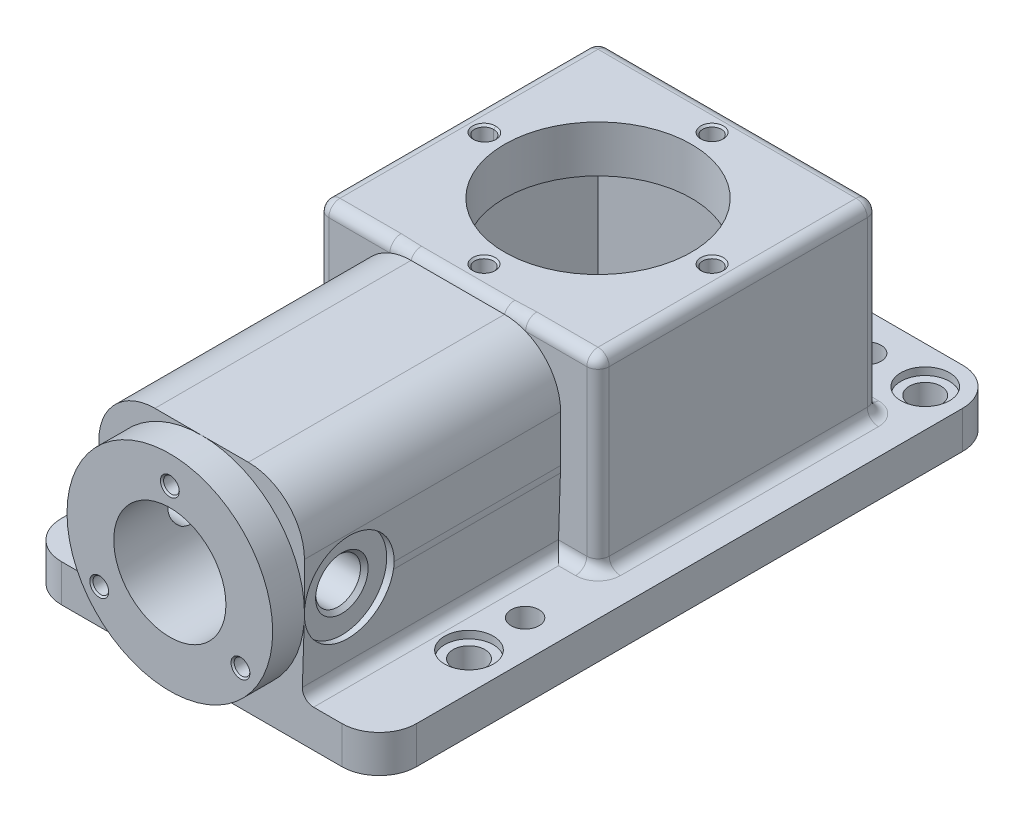
from build123d import *

# Parameters (mm, degrees)
SKETCH1_R                       = 27.5
BOSS_EXTRUDE1_DEPTH             = 77
SKETCH2_W                       = 75
SKETCH2_H                       = 56.897365196
BOSS_EXTRUDE2_DEPTH             = 75
SKETCH3_R                       = 15
CUT_EXTRUDE1_DEPTH              = 105
SKETCH4_R                       = 25
CUT_EXTRUDE2_DEPTH              = 17
SKETCH5_R                       = 21
CUT_EXTRUDE3_DEPTH              = 65
CUT_EXTRUDE4_START              = -12.5
SKETCH6_W                       = 63
SKETCH6_H                       = 63
CUT_EXTRUDE4_DEPTH              = 39.5
SKETCH7_R                       = 25
SKETCH7_R_2                     = 21
BOSS_EXTRUDE3_DEPTH             = 2
BOSS_EXTRUDE4_DEPTH             = 47.5
BOSS_EXTRUDE5_START             = -68.5
BOSS_EXTRUDE5_DEPTH             = 68.5
FILLET1_R                       = 15
FILLET2_R                       = 3
BOSS_EXTRUDE7_REACH             = 124.474
SKETCH19_W                      = 17.5
SKETCH19_H                      = 130
SKETCH20_W                      = 148
SKETCH20_H                      = 3.566
CUT_EXTRUDE9_DEPTH              = 205
SKETCH10_R                      = 6.5
CUT_EXTRUDE5_DEPTH              = 2
SKETCH11_R                      = 4.25
CUT_EXTRUDE6_DEPTH              = 69
FILLET3_R                       = 10
SKETCH12_R                      = 21
CUT_EXTRUDE7_DEPTH              = 69
BOSS_EXTRUDE6_START             = 2
SKETCH13_R                      = 25
SKETCH13_R_2                    = 21
BOSS_EXTRUDE6_DEPTH             = 2
CIRPATTERN1_COUNT               = 3
SKETCH16_R                      = 3.735111871
SKETCH16_R_2                    = 3.711892177
CUT_EXTRUDE8_DEPTH              = 25
FILLET4_R                       = 3
SKETCH22_R                      = 12
CUT_EXTRUDE10_DEPTH             = 2
M6_TAPPED_HOLE1_D               = 5
M6_TAPPED_HOLE1_DEPTH           = 9.497848452
M6_TAPPED_HOLE1_CSINK_D         = 6.05
M6_TAPPED_HOLE1_CSINK_ANGLE     = 90
M6_TAPPED_HOLE1_TIP             = 1.502151548
SKETCH30_R                      = 7
CUT_EXTRUDE11_DEPTH             = 1
M8X1_0_TAPPED_HOLE1_D           = 7
M8X1_0_TAPPED_HOLE1_DEPTH       = 16.896987833
M8X1_0_TAPPED_HOLE1_CSINK_D     = 8.05
M8X1_0_TAPPED_HOLE1_CSINK_ANGLE = 90
M8X1_0_TAPPED_HOLE1_TIP         = 2.103012167


with BuildPart() as part:
    # Sketch1 → Boss-Extrude1 (new body)
    with BuildSketch(Plane.XY):
        Circle(SKETCH1_R)
    extrude(amount=BOSS_EXTRUDE1_DEPTH)

    # Sketch2 → Boss-Extrude2 (add)
    with BuildSketch(Plane(origin=(0, 0, 0), x_dir=(-1, 0, 0), z_dir=(0, 0, -1))):
        with Locations((0, 0.948682598)):
            Rectangle(SKETCH2_W, SKETCH2_H)
    extrude(amount=BOSS_EXTRUDE2_DEPTH)

    # Sketch3 → Cut-Extrude1 (cut)
    with BuildSketch(Plane.XY.offset(77)):
        Circle(SKETCH3_R)
    extrude(amount=-CUT_EXTRUDE1_DEPTH, mode=Mode.SUBTRACT)

    # Sketch4 → Cut-Extrude2 (cut)
    with BuildSketch(Plane(origin=(0, 29.397365196, 0), x_dir=(1, 0, 0), z_dir=(0, 1, 0))):
        with Locations(Location((0, 37.5, 0), (0, 0, 180))):
            Circle(SKETCH4_R)
    extrude(amount=-CUT_EXTRUDE2_DEPTH, mode=Mode.SUBTRACT)

    # Sketch5 → Cut-Extrude3 (cut)
    with BuildSketch(Plane.XZ.offset(27.5)):
        with Locations(Location((0, -37.5, 0), (0, 0, 270))):
            Circle(SKETCH5_R)
    extrude(amount=-CUT_EXTRUDE3_DEPTH, mode=Mode.SUBTRACT)

    # Sketch6 → Cut-Extrude4 (cut)
    with BuildSketch(Plane(origin=(0, 29.397365196, 0), x_dir=(1, 0, 0), z_dir=(0, 1, 0)).offset(CUT_EXTRUDE4_START)):
        with Locations((0, 37.5)):
            Rectangle(SKETCH6_W, SKETCH6_H)
    extrude(amount=-CUT_EXTRUDE4_DEPTH, mode=Mode.SUBTRACT)

    # Sketch7 → Boss-Extrude3 (add)
    with BuildSketch(Plane(origin=(0, -22.602634804, 0), x_dir=(1, 0, 0), z_dir=(0, 1, 0))):
        with Locations(Location((0, 37.5, 0), (0, 0, 180))):
            Circle(SKETCH7_R)
        with Locations(Location((0, 37.5, 0), (0, 0, 90))):
            Circle(SKETCH7_R_2, mode=Mode.SUBTRACT)
    extrude(amount=BOSS_EXTRUDE3_DEPTH)

    # Sketch8 → Boss-Extrude4 (add, symmetric)
    with BuildSketch(Plane(origin=(0, 0, 0), x_dir=(0, 0, -1), z_dir=(1, 0, 0))):
        Polygon((-68.5, -20.5), (97.5, -20.5), (97.5, -30.5), (79.5, -30.5), (79.5, -27.5), (-50.5, -27.5), (-50.5, -34.066), (-68.5, -34.066), align=None)
    extrude(amount=BOSS_EXTRUDE4_DEPTH, both=True)

    # Sketch9 → Boss-Extrude5 (add)
    with BuildSketch(Plane.XY.offset(68.5).offset(BOSS_EXTRUDE5_START)):
        with BuildLine():
            Line((-27.5, 27.5), (-27.5, 0))
            ThreePointArc((-27.5, 0), (-19.445436463, 19.445436502), (5.5e-08, 27.5))
            Line((5.5e-08, 27.5), (-27.5, 27.5))
        make_face()
        with BuildLine():
            ThreePointArc((-18.33030278, -20.5), (-25.103120587, -11.228683662), (-27.5, 0))
            Line((-27.5, 0), (-27.5, -20.5))
            Line((-27.5, -20.5), (-18.33030278, -20.5))
        make_face()
        with BuildLine():
            Line((27.5, 27.5), (5.5e-08, 27.5))
            ThreePointArc((5.5e-08, 27.5), (19.445436502, 19.445436463), (27.5, 0))
            Line((27.5, 0), (27.5, 27.5))
        make_face()
        with BuildLine():
            Line((26.841682092, -20.5), (27.443339726, -1.764399243))
            ThreePointArc((27.443339726, -1.764399243), (24.729785098, -12.028621243), (18.33030278, -20.5))
            Line((18.33030278, -20.5), (26.841682092, -20.5))
        make_face()
    extrude(amount=BOSS_EXTRUDE5_DEPTH)

    # Fillet1
    fillet1_edges = [part.edges().sort_by_distance(p)[0] for p in [
        (-27.5, 27.5, 34.25),
        (27.5, 27.5, 34.25),
    ]]
    fillet(fillet1_edges, radius=FILLET1_R)

    # Fillet2
    fillet2_edges = [part.edges().sort_by_distance(p)[0] for p in [
        (-32.5, -20.5, 0),
        (-27.5, -20.5, 34.25),
        (26.841682092, -20.5, 34.25),
        (0, 29.397365196, 0),
        (-37.5, 29.397365196, -37.5),
        (37.5, 4.448682598, 0),
        (-37.5, 4.448682598, 0),
        (-37.5, 4.448682598, -75),
        (37.5, 29.397365196, -37.5),
        (32.170841046, -20.5, 0),
        (-37.5, -20.5, -37.5),
        (37.5, -20.5, -37.5),
        (0, -20.5, -75),
        (0, 29.397365196, -75),
        (37.5, 4.448682598, -75),
    ]]
    fillet(fillet2_edges, radius=FILLET2_R)

    # Boss-Extrude7: up to this face of the body (flat: up to its plane)
    boss_extrude7_end = Plane(part.part.faces().sort_by_distance((0, -34.066, 59.5))[0])
    # Sketch19 → Boss-Extrude7 (add, up to the picked face)
    with BuildSketch(Plane.XZ.offset(27.5), mode=Mode.PRIVATE) as boss_extrude7_sk1:
        with Locations((-38.75, -14.5)):
            Rectangle(SKETCH19_W, SKETCH19_H)
    boss_extrude7_tool1 = split(extrude(boss_extrude7_sk1.sketch, amount=BOSS_EXTRUDE7_REACH, mode=Mode.PRIVATE), bisect_by=boss_extrude7_end, keep=Keep.BOTH, mode=Mode.PRIVATE)
    # Sketch19 → Boss-Extrude7 (add, up to the picked face)
    with BuildSketch(Plane.XZ.offset(27.5), mode=Mode.PRIVATE) as boss_extrude7_sk2:
        with Locations((38.75, -14.5)):
            Rectangle(SKETCH19_W, SKETCH19_H)
    boss_extrude7_tool2 = split(extrude(boss_extrude7_sk2.sketch, amount=BOSS_EXTRUDE7_REACH, mode=Mode.PRIVATE), bisect_by=boss_extrude7_end, keep=Keep.BOTH, mode=Mode.PRIVATE)
    add(boss_extrude7_tool1.solids().sort_by(Axis((-38.75, -27.5, -14.5), (0, -1, 0)))[0])
    add(boss_extrude7_tool2.solids().sort_by(Axis((38.75, -27.5, -14.5), (0, -1, 0)))[0])

    # Sketch20 → Cut-Extrude9 (cut)
    with BuildSketch(Plane(origin=(47.5, 0, 0), x_dir=(0, 0, -1), z_dir=(1, 0, 0))):
        with Locations((5.5, -32.283)):
            Rectangle(SKETCH20_W, SKETCH20_H)
    extrude(amount=-CUT_EXTRUDE9_DEPTH, mode=Mode.SUBTRACT)

    # Sketch10 → Cut-Extrude5 (cut)
    with BuildSketch(Plane(origin=(0, -20.5, 0), x_dir=(1, 0, 0), z_dir=(0, 1, 0))):
        with Locations(Location((37.5, 87.5, 0), (0, 0, 270))):
            Circle(SKETCH10_R)
        with Locations(Location((-37.5, 87.5, 0), (0, 0, 270))):
            Circle(SKETCH10_R)
        with Locations(Location((-37.5, -34.5, 0), (0, 0, 270))):
            Circle(SKETCH10_R)
        with Locations(Location((37.5, -34.5, 0), (0, 0, 270))):
            Circle(SKETCH10_R)
    extrude(amount=-CUT_EXTRUDE5_DEPTH, mode=Mode.SUBTRACT)

    # Sketch11 → Cut-Extrude6 (cut)
    with BuildSketch(Plane(origin=(0, -22.5, 0), x_dir=(1, 0, 0), z_dir=(0, 1, 0))):
        with Locations(Location((-37.5, 87.5, 0), (0, 0, 270))):
            Circle(SKETCH11_R)
        with Locations(Location((37.5, 87.5, 0), (0, 0, 270))):
            Circle(SKETCH11_R)
        with Locations(Location((-37.5, -34.5, 0), (0, 0, 270))):
            Circle(SKETCH11_R)
        with Locations(Location((37.5, -34.5, 0), (0, 0, 270))):
            Circle(SKETCH11_R)
    extrude(amount=-CUT_EXTRUDE6_DEPTH, mode=Mode.SUBTRACT)

    # Fillet3
    fillet3_edges = [part.edges().sort_by_distance(p)[0] for p in [
        (-47.5, -25.5, -97.5),
        (-47.5, -25.5, 68.5),
        (47.5, -25.5, -97.5),
        (47.5, -25.5, 68.5),
    ]]
    fillet(fillet3_edges, radius=FILLET3_R)

    # Sketch12 → Cut-Extrude7 (cut)
    with BuildSketch(Plane(origin=(0, 29.397365196, 0), x_dir=(1, 0, 0), z_dir=(0, 1, 0))):
        with Locations(Location((0, 37.5, 0), (0, 0, 90))):
            Circle(SKETCH12_R)
    extrude(amount=-CUT_EXTRUDE7_DEPTH, mode=Mode.SUBTRACT)

    # Sketch13 → Boss-Extrude6 (add)
    with BuildSketch(Plane(origin=(0, -20.5, 0), x_dir=(1, 0, 0), z_dir=(0, 1, 0)).offset(BOSS_EXTRUDE6_START)):
        with Locations(Location((0, 37.5, 0), (0, 0, 180))):
            Circle(SKETCH13_R)
        with Locations(Location((0, 37.5, 0), (0, 0, 270))):
            Circle(SKETCH13_R_2, mode=Mode.SUBTRACT)
    extrude(amount=-BOSS_EXTRUDE6_DEPTH)

    # Sketch15 → M5 Tapped Hole1 (revolve, cut)
    with BuildSketch(Plane(origin=(0, 20, 77), x_dir=(0, -1, 0), z_dir=(1, 0, 0))):
        Polygon((0, 0), (0, 11), (2.1, 9.7381927), (2.1, 0.425), (2.525, 0), align=None)
    m5_tapped_hole1 = revolve(axis=Axis((0, 20, 83.35), (0, 0, -1)), mode=Mode.SUBTRACT)

    # CirPattern1: M5 Tapped Hole1 ×3 about axis
    cirpattern1_axis = Axis((0, -1.801317402, 0), (0, 0, 1))
    for i in range(1, CIRPATTERN1_COUNT):
        add(m5_tapped_hole1.rotate(cirpattern1_axis, i * 360 / CIRPATTERN1_COUNT), mode=Mode.SUBTRACT)

    # Sketch16 → Cut-Extrude8 (cut)
    with BuildSketch(Plane(origin=(0, -20.5, 0), x_dir=(1, 0, 0), z_dir=(0, 1, 0))):
        with Locations(Location((37.5, -19.5, 0), (0, 0, 270))):
            Circle(SKETCH16_R)
        with Locations(Location((22, 87.5, 0), (0, 0, 270))):
            Circle(SKETCH16_R_2)
    extrude(amount=-CUT_EXTRUDE8_DEPTH, mode=Mode.SUBTRACT)

    # Fillet4
    fillet4_edges = [part.edges().sort_by_distance(p)[0] for p in [
        (-30, -29, -79.5),
        (30, -29, -79.5),
        (-30, -29, 50.5),
        (30, -29, 50.5),
    ]]
    fillet(fillet4_edges, radius=FILLET4_R)

    # Sketch22 → Cut-Extrude10 (cut)
    with BuildSketch(Plane.ZY.offset(27.5)):
        with Locations(Location((56.5, 0, 0), (0, 0, 270))):
            Circle(SKETCH22_R)
    cut_extrude10 = extrude(amount=-CUT_EXTRUDE10_DEPTH, mode=Mode.SUBTRACT)

    # Sketch25 → M14 Tapped Hole1 (revolve, cut)
    with BuildSketch(Plane(origin=(-25.5, 0, 56.5), x_dir=(0, 0, 1), z_dir=(0, 1, 0))):
        Polygon((0, 0), (0, 15), (6, 11.394836286), (6, 1.025), (7.025, 0), align=None)
    m14_tapped_hole1 = revolve(axis=Axis((-31.85, 0, 56.5), (1, 0, 0)), mode=Mode.SUBTRACT)

    # Mirror1: Cut-Extrude10, M14 Tapped Hole1 across plane
    add(cut_extrude10.mirror(Plane(origin=(0, 0, 0), x_dir=(0, 0, 1), z_dir=(1, 0, 0))), mode=Mode.SUBTRACT)
    add(m14_tapped_hole1.mirror(Plane(origin=(0, 0, 0), x_dir=(0, 0, 1), z_dir=(1, 0, 0))), mode=Mode.SUBTRACT)

    # M6 Tapped Hole1
    with Locations(Plane(origin=(0, 29.397365196, 0), x_dir=(1, 0, 0), z_dir=(0, 1, 0))):
        with Locations((0, 68), (30.5, 37.5), (0, 7), (-30.5, 37.5), (-30.286228554, 37.5)):
            CounterSinkHole(M6_TAPPED_HOLE1_D / 2, M6_TAPPED_HOLE1_CSINK_D / 2, depth=M6_TAPPED_HOLE1_DEPTH, counter_sink_angle=M6_TAPPED_HOLE1_CSINK_ANGLE)
            with Locations((0, 0, -(M6_TAPPED_HOLE1_DEPTH + M6_TAPPED_HOLE1_TIP / 2))):  # 118° drill point
                Cone(0, M6_TAPPED_HOLE1_D / 2, M6_TAPPED_HOLE1_TIP, mode=Mode.SUBTRACT)

    # Sketch30 → Cut-Extrude11 (cut)
    with BuildSketch(Plane.ZY.offset(37.5)):
        with Locations((-18, 0)):
            Circle(SKETCH30_R)
    extrude(amount=-CUT_EXTRUDE11_DEPTH, mode=Mode.SUBTRACT)

    # M8x1.0 Tapped Hole1
    with Locations(Plane.ZY.offset(36.5)):
        with Locations((-18, 0)):
            CounterSinkHole(M8X1_0_TAPPED_HOLE1_D / 2, M8X1_0_TAPPED_HOLE1_CSINK_D / 2, depth=M8X1_0_TAPPED_HOLE1_DEPTH, counter_sink_angle=M8X1_0_TAPPED_HOLE1_CSINK_ANGLE)
            with Locations((0, 0, -(M8X1_0_TAPPED_HOLE1_DEPTH + M8X1_0_TAPPED_HOLE1_TIP / 2))):  # 118° drill point
                Cone(0, M8X1_0_TAPPED_HOLE1_D / 2, M8X1_0_TAPPED_HOLE1_TIP, mode=Mode.SUBTRACT)


solid = part.part
